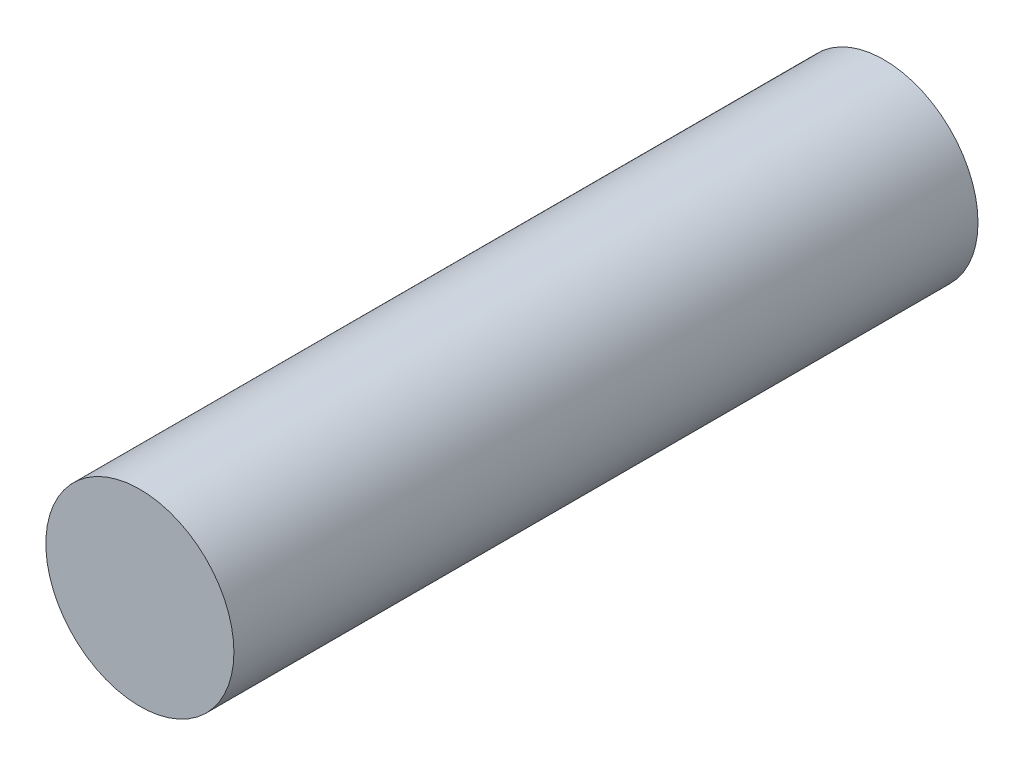
SolidWorks part; units mm, degrees
ref_plane "前视基准面" through (0, 0, 0) normal (0, 0, 1) x (1, 0, 0)
ref_plane "上视基准面" through (0, 0, 0) normal (0, 1, 0) x (1, 0, 0)
ref_plane "右视基准面" through (0, 0, 0) normal (1, 0, 0) x (0, 0, -1)
sketch "草图1" plane through (0, 0, 0) normal (0, 0, 1) x (1, 0, 0)
  circle A0 centre (0, 0) radius 1.15
  dimension "D1" = 2.3
extrude "凸台-拉伸1" add sketch "草图1" along normal blind 9.1
